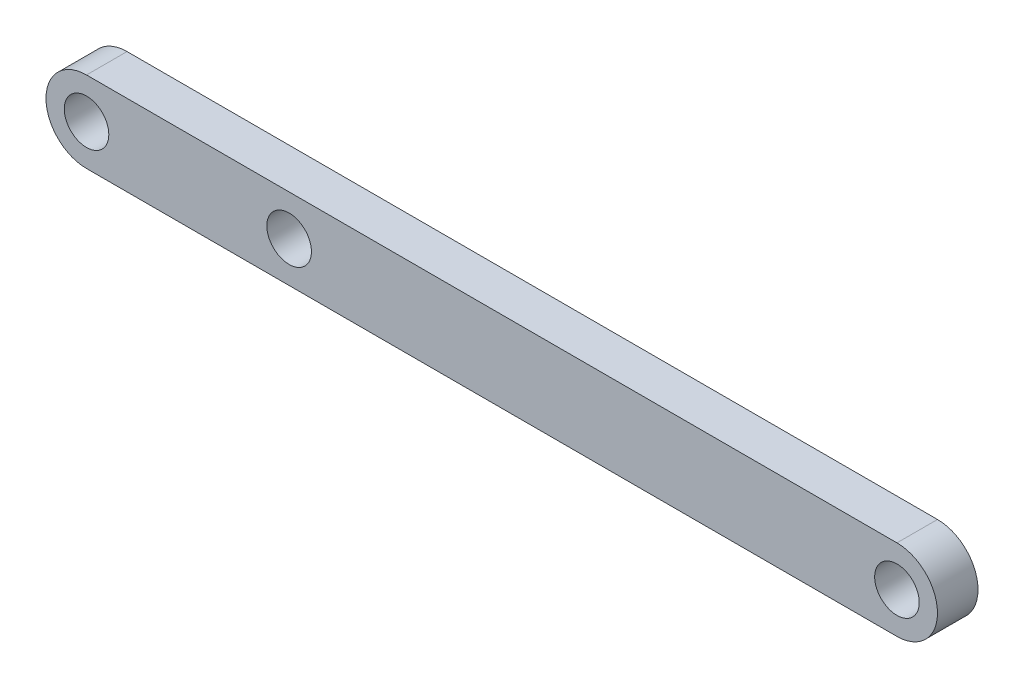
from build123d import *

# Parameters (mm, degrees)
SKETCH1_R           = 0.55
THIGH1_LENGTH_DEPTH = 0.5


with BuildPart() as part:
    # Sketch1 → Thigh1 length (new, symmetric)
    with BuildSketch(Plane.XY):
        with BuildLine():
            Line((-10, 1), (10, 1))
            ThreePointArc((10, 1), (11, 0), (10, -1))
            Line((10, -1), (-10, -1))
            ThreePointArc((-10, -1), (-11, 0), (-10, 1))
        make_face()
        with Locations((-10, 0)):
            Circle(SKETCH1_R, mode=Mode.SUBTRACT)
        with Locations((10, 0)):
            Circle(SKETCH1_R, mode=Mode.SUBTRACT)
        with Locations((-5, 0)):
            Circle(SKETCH1_R, mode=Mode.SUBTRACT)
    extrude(amount=THIGH1_LENGTH_DEPTH, both=True)


solid = part.part
